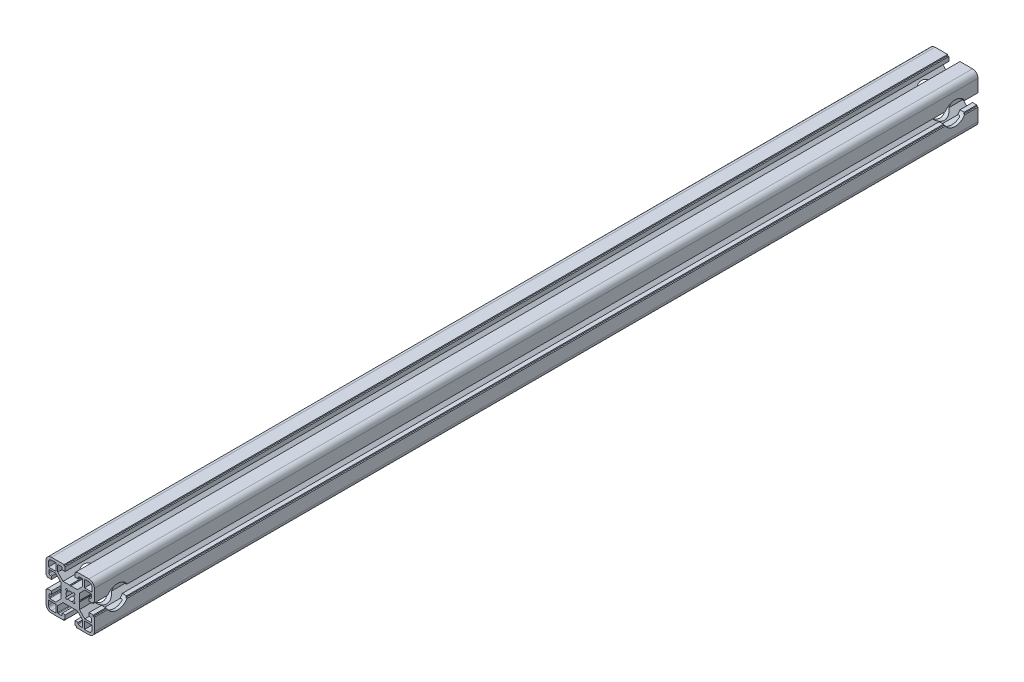
from build123d import *

# Parameters (mm, degrees)
EXTRUDE_1_DEPTH         = 730
HOLE_WIZARD_19_0_19_1_D = 19


with BuildPart() as part:
    # 草图1 → 凸台-拉伸1 (new body)
    with BuildSketch(Plane.XY):
        with BuildLine():
            Line((-18.9995, -4.100341675), (-18.9995, -5.100341675))
            Line((-18.9995, -5.100341675), (-19.9995, -5.100341675))
            Line((-19.9995, -5.100341675), (-19.9995, -15.500341675))
            ThreePointArc((-19.9995, -15.500341675), (-18.681480515, -18.682322191), (-15.4995, -20.000341675))
            Line((-15.4995, -20.000341675), (-5.0995, -20.000341675))
            Line((-5.0995, -20.000341675), (-5.0995, -19.000341675))
            Line((-5.0995, -19.000341675), (-4.0995, -19.000341675))
            Line((-4.0995, -19.000341675), (-4.0995, -15.500341675))
            Line((-4.0995, -15.500341675), (-6.5995, -15.500341675))
            Line((-6.5995, -15.500341675), (-6.5995, -16.500341675))
            ThreePointArc((-6.5995, -16.500341675), (-6.892393219, -17.207448457), (-7.5995, -17.500341675))
            Line((-7.5995, -17.500341675), (-9.7995, -17.500341675))
            ThreePointArc((-9.7995, -17.500341675), (-10.153053391, -17.353895066), (-10.2995, -17.000341675))
            Line((-10.2995, -17.000341675), (-10.2995, -11.997341675))
            Line((-10.2995, -11.997341675), (-5.9025, -7.600341675))
            Line((-5.9025, -7.600341675), (-0.5195, -7.600341675))
            Line((-0.5195, -7.600341675), (0.0005, -7.300341675))
            Line((0.0005, -7.300341675), (0.5195, -7.600341675))
            Line((0.5195, -7.600341675), (5.9035, -7.600341675))
            Line((5.9035, -7.600341675), (10.3005, -11.997341675))
            Line((10.3005, -11.997341675), (10.3005, -17.000341675))
            ThreePointArc((10.3005, -17.000341675), (10.154053391, -17.353895066), (9.8005, -17.500341675))
            Line((9.8005, -17.500341675), (7.6005, -17.500341675))
            ThreePointArc((7.6005, -17.500341675), (6.893393219, -17.207448457), (6.6005, -16.500341675))
            Line((6.6005, -16.500341675), (6.6005, -15.500341675))
            Line((6.6005, -15.500341675), (4.1005, -15.500341675))
            Line((4.1005, -15.500341675), (4.1005, -19.000341675))
            Line((4.1005, -19.000341675), (5.1005, -19.000341675))
            Line((5.1005, -19.000341675), (5.1005, -20.000341675))
            Line((5.1005, -20.000341675), (15.5005, -20.000341675))
            ThreePointArc((15.5005, -20.000341675), (18.682480515, -18.682322191), (20.0005, -15.500341675))
            Line((20.0005, -15.500341675), (20.0005, -5.100341675))
            Line((20.0005, -5.100341675), (19.0005, -5.100341675))
            Line((19.0005, -5.100341675), (19.0005, -4.100341675))
            Line((19.0005, -4.100341675), (15.5005, -4.100341675))
            Line((15.5005, -4.100341675), (15.5005, -6.600341675))
            Line((15.5005, -6.600341675), (16.5005, -6.600341675))
            ThreePointArc((16.5005, -6.600341675), (17.207606781, -6.893234894), (17.5005, -7.600341675))
            Line((17.5005, -7.600341675), (17.5005, -9.800341675))
            ThreePointArc((17.5005, -9.800341675), (17.354053391, -10.153895066), (17.0005, -10.300341675))
            Line((17.0005, -10.300341675), (11.9975, -10.300341675))
            Line((11.9975, -10.300341675), (7.6005, -5.903341675))
            Line((7.6005, -5.903341675), (7.6005, -0.520341675))
            Line((7.6005, -0.520341675), (7.3005, -0.000341675))
            Line((7.3005, -0.000341675), (7.6005, 0.519658325))
            Line((7.6005, 0.519658325), (7.6005, 5.902658325))
            Line((7.6005, 5.902658325), (11.9975, 10.299658325))
            Line((11.9975, 10.299658325), (17.0005, 10.299658325))
            ThreePointArc((17.0005, 10.299658325), (17.354053391, 10.153211715), (17.5005, 9.799658325))
            Line((17.5005, 9.799658325), (17.5005, 7.599658325))
            ThreePointArc((17.5005, 7.599658325), (17.207606781, 6.892551543), (16.5005, 6.599658325))
            Line((16.5005, 6.599658325), (15.5005, 6.599658325))
            Line((15.5005, 6.599658325), (15.5005, 4.099658325))
            Line((15.5005, 4.099658325), (19.0005, 4.099658325))
            Line((19.0005, 4.099658325), (19.0005, 5.099658325))
            Line((19.0005, 5.099658325), (20.0005, 5.099658325))
            Line((20.0005, 5.099658325), (20.0005, 15.499658325))
            ThreePointArc((20.0005, 15.499658325), (18.682480515, 18.68163884), (15.5005, 19.999658325))
            Line((15.5005, 19.999658325), (5.1005, 19.999658325))
            Line((5.1005, 19.999658325), (5.1005, 18.999658325))
            Line((5.1005, 18.999658325), (4.1005, 18.999658325))
            Line((4.1005, 18.999658325), (4.1005, 15.499658325))
            Line((4.1005, 15.499658325), (6.6005, 15.499658325))
            ThreePointArc((6.6005, 15.499658325), (6.393348977, 15.999658325), (6.6005, 16.499658325))
            ThreePointArc((6.6005, 16.499658325), (6.893393219, 17.206765106), (7.6005, 17.499658325))
            Line((7.6005, 17.499658325), (9.8005, 17.499658325))
            ThreePointArc((9.8005, 17.499658325), (10.154053391, 17.353211715), (10.3005, 16.999658325))
            Line((10.3005, 16.999658325), (10.3005, 11.996658325))
            Line((10.3005, 11.996658325), (5.9035, 7.599658325))
            Line((5.9035, 7.599658325), (0.5195, 7.599658325))
            Line((0.5195, 7.599658325), (0.0005, 7.299658325))
            Line((0.0005, 7.299658325), (-0.5195, 7.599658325))
            Line((-0.5195, 7.599658325), (-5.9025, 7.599658325))
            Line((-5.9025, 7.599658325), (-10.2995, 11.996658325))
            Line((-10.2995, 11.996658325), (-10.2995, 16.999658325))
            ThreePointArc((-10.2995, 16.999658325), (-10.153053391, 17.353211715), (-9.7995, 17.499658325))
            Line((-9.7995, 17.499658325), (-7.5995, 17.499658325))
            ThreePointArc((-7.5995, 17.499658325), (-6.892393219, 17.206765106), (-6.5995, 16.499658325))
            Line((-6.5995, 16.499658325), (-6.5995, 15.499658325))
            Line((-6.5995, 15.499658325), (-4.0995, 15.499658325))
            Line((-4.0995, 15.499658325), (-4.0995, 18.999658325))
            Line((-4.0995, 18.999658325), (-5.0995, 18.999658325))
            Line((-5.0995, 18.999658325), (-5.0995, 19.999658325))
            Line((-5.0995, 19.999658325), (-15.4995, 19.999658325))
            ThreePointArc((-15.4995, 19.999658325), (-18.681480515, 18.68163884), (-19.9995, 15.499658325))
            Line((-19.9995, 15.499658325), (-19.9995, 5.099658325))
            Line((-19.9995, 5.099658325), (-18.9995, 5.099658325))
            Line((-18.9995, 5.099658325), (-18.9995, 4.099658325))
            Line((-18.9995, 4.099658325), (-15.4995, 4.099658325))
            Line((-15.4995, 4.099658325), (-15.4995, 6.599658325))
            Line((-15.4995, 6.599658325), (-16.4995, 6.599658325))
            ThreePointArc((-16.4995, 6.599658325), (-17.206606781, 6.892551543), (-17.4995, 7.599658325))
            Line((-17.4995, 7.599658325), (-17.4995, 9.799658325))
            ThreePointArc((-17.4995, 9.799658325), (-17.353053391, 10.153211715), (-16.9995, 10.299658325))
            Line((-16.9995, 10.299658325), (-11.9965, 10.299658325))
            Line((-11.9965, 10.299658325), (-7.5995, 5.902658325))
            Line((-7.5995, 5.902658325), (-7.5995, 0.519658325))
            Line((-7.5995, 0.519658325), (-7.2995, -0.000341675))
            Line((-7.2995, -0.000341675), (-7.5995, -0.520341675))
            Line((-7.5995, -0.520341675), (-7.5995, -5.903341675))
            Line((-7.5995, -5.903341675), (-11.9965, -10.300341675))
            Line((-11.9965, -10.300341675), (-16.9995, -10.300341675))
            ThreePointArc((-16.9995, -10.300341675), (-17.353053391, -10.153895066), (-17.4995, -9.800341675))
            Line((-17.4995, -9.800341675), (-17.4995, -7.600341675))
            ThreePointArc((-17.4995, -7.600341675), (-17.206606781, -6.893234894), (-16.4995, -6.600341675))
            Line((-16.4995, -6.600341675), (-15.4995, -6.600341675))
            Line((-15.4995, -6.600341675), (-15.4995, -4.100341675))
            Line((-15.4995, -4.100341675), (-18.9995, -4.100341675))
        make_face()
        with BuildLine():
            Line((15.5005, -18.000341675), (11.8005, -18.000341675))
            Line((11.8005, -18.000341675), (11.8005, -11.800341675))
            Line((11.8005, -11.800341675), (18.0005, -11.800341675))
            Line((18.0005, -11.800341675), (18.0005, -15.500341675))
            ThreePointArc((18.0005, -15.500341675), (17.268266953, -17.268108628), (15.5005, -18.000341675))
        make_face(mode=Mode.SUBTRACT)
        with BuildLine():
            Line((18.0005, 11.799658325), (11.8005, 11.799658325))
            Line((11.8005, 11.799658325), (11.8005, 17.999658325))
            Line((11.8005, 17.999658325), (15.5005, 17.999658325))
            ThreePointArc((15.5005, 17.999658325), (17.268266953, 17.267425278), (18.0005, 15.499658325))
            Line((18.0005, 15.499658325), (18.0005, 11.799658325))
        make_face(mode=Mode.SUBTRACT)
        with BuildLine():
            Line((-1.8145, -2.875341675), (-3.004391671, -4.066450004))
            Line((-3.004391671, -4.066450004), (-4.065608329, -3.005233346))
            Line((-4.065608329, -3.005233346), (-2.8745, -1.815341675))
            ThreePointArc((-2.8745, -1.815341675), (-3.399473913, -0.000341675), (-2.8745, 1.814658325))
            Line((-2.8745, 1.814658325), (-4.064391671, 3.005766654))
            Line((-4.064391671, 3.005766654), (-3.004391671, 4.065766654))
            Line((-3.004391671, 4.065766654), (-1.8145, 2.874658325))
            ThreePointArc((-1.8145, 2.874658325), (0, 3.399316649), (1.8145, 2.874658325))
            Line((1.8145, 2.874658325), (3.0055, 4.065658325))
            Line((3.0055, 4.065658325), (4.066608329, 3.004549996))
            Line((4.066608329, 3.004549996), (2.8755, 1.814658325))
            ThreePointArc((2.8755, 1.814658325), (3.400473913, -0.000341675), (2.8755, -1.815341675))
            Line((2.8755, -1.815341675), (4.066608329, -3.005233346))
            Line((4.066608329, -3.005233346), (3.0055, -4.066341675))
            Line((3.0055, -4.066341675), (1.8145, -2.875341675))
            ThreePointArc((1.8145, -2.875341675), (0, -3.4), (-1.8145, -2.875341675))
        make_face(mode=Mode.SUBTRACT)
        with BuildLine():
            Line((-17.9995, -15.500341675), (-17.9995, -11.800341675))
            Line((-17.9995, -11.800341675), (-11.7995, -11.800341675))
            Line((-11.7995, -11.800341675), (-11.7995, -18.000341675))
            Line((-11.7995, -18.000341675), (-15.4995, -18.000341675))
            ThreePointArc((-15.4995, -18.000341675), (-17.267266953, -17.268108628), (-17.9995, -15.500341675))
        make_face(mode=Mode.SUBTRACT)
        with BuildLine():
            Line((-11.7995, 17.999658325), (-11.7995, 11.799658325))
            Line((-11.7995, 11.799658325), (-17.9995, 11.799658325))
            Line((-17.9995, 11.799658325), (-17.9995, 15.499658325))
            ThreePointArc((-17.9995, 15.499658325), (-17.267266953, 17.267425278), (-15.4995, 17.999658325))
            Line((-15.4995, 17.999658325), (-11.7995, 17.999658325))
        make_face(mode=Mode.SUBTRACT)
    extrude(amount=-EXTRUDE_1_DEPTH)

    # Ø19.0 (19) 直径孔1 (through all)
    with Locations(Plane(origin=(-19.9995, -0.000841675, 0), x_dir=(0, -1, 0), z_dir=(-1, 0, 0))):
        with Locations((-0.0005, -19), (-0.0005, -711)):
            Hole(HOLE_WIZARD_19_0_19_1_D / 2)


solid = part.part
